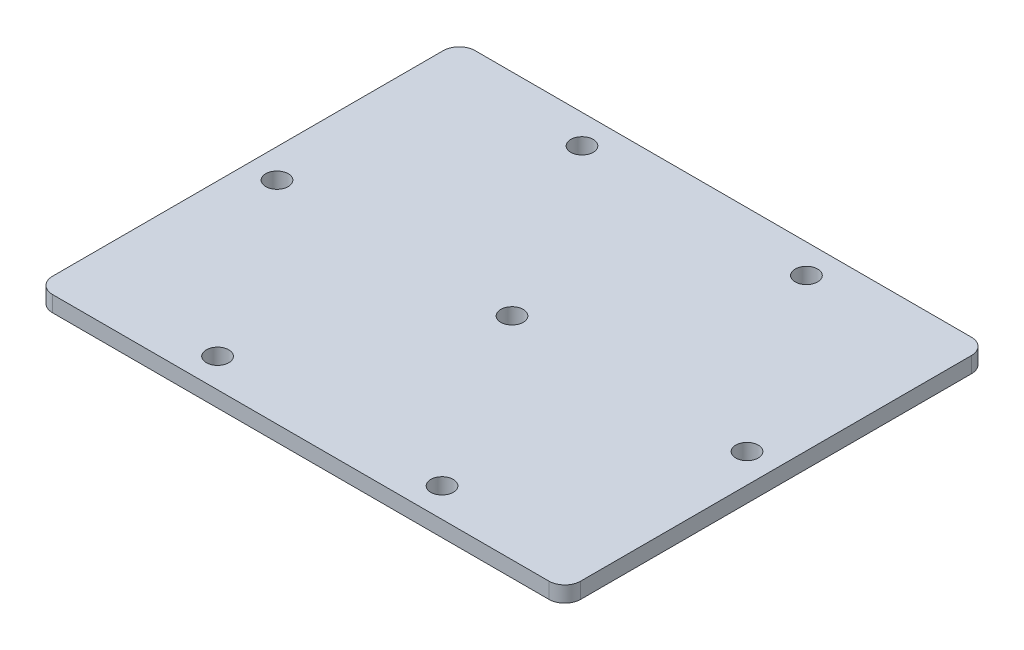
SolidWorks part; units mm, degrees
ref_plane "Front Plane" through (0, 0, 0) normal (0, 0, 1) x (1, 0, 0)
ref_plane "Top Plane" through (0, 0, 0) normal (0, 1, 0) x (1, 0, 0)
ref_plane "Right Plane" through (0, 0, 0) normal (1, 0, 0) x (0, 0, -1)
other "Configuration Table"
sketch "Sketch1" plane through (0, 0, 0) normal (0, 1, 0) x (1, 0, 0)
  line L1 (-100, -80) -> (100, -80)
  line L2 (-100, -80) -> (-100, 80)
  line L3 (-100, 80) -> (100, 80)
  line L4 (100, -80) -> (100, 80)
  line L5 (-100, -80) -> (100, 80) construction
  line L6 (-100, 80) -> (100, -80) construction
  point P0 (0, 0)
  dimension "D1" = 160
  dimension "D2" = 200
extrude "Boss-Extrude1" add sketch "Sketch1" along normal blind 6
fillet "Fillet1" radius 6 4 edges at (-100, 3, -80) (100, 3, -80) (100, 3, 80) (-100, 3, 80)
sketch "Sketch2" plane through (0, 6, 0) normal (0, 1, 0) x (1, 0, 0)
  line L0 (-138.2328, 0) -> (159.8736, 0) construction
  line L1 (0, 96.9307) -> (0, -97.5346) construction
  circle A0 centre (0, 0) radius 7.5
  circle A1 centre (-42.5, 69) radius 7.5
  circle A2 centre (42.5, 69) radius 7.5
  circle A3 centre (-89, 0) radius 7.5
  circle A4 centre (89, 0) radius 7.5
  circle A5 centre (-42.5, -69) radius 7.5
  circle A6 centre (42.5, -69) radius 7.5
  dimension "D1" = 15
  dimension "D2" = 15
  dimension "D3" = 15
  dimension "D4" = 15
  dimension "D5" = 15
  dimension "D6" = 15
  dimension "D7" = 15
  dimension "D8" = 85
  dimension "D9" = 138
  dimension "D10" = 178
hole_wizard "M10 Tapped Hole1" positions "Sketch3" profile "Sketch4" tap size "M10" standard "GB" end condition through all
sketch "Sketch3" plane through (0, 6, 0) normal (0, 1, 0) x (1, 0, 0)
  point P0 (0, 0)
  point P3 (42.5, 69)
  point P6 (-42.5, 69)
  point P9 (-89, 0)
  point P12 (89, 0)
  point P15 (42.5, -69)
  point P18 (-42.5, -69)
sketch "Sketch4" plane through (0, 6, 0) normal (1, 0, 0) x (0, 0, 1)
  line L0 (0, 0) -> (0, 6)
  line L1 (0, 6) -> (4.25, 6)
  line L2 (4.25, 6) -> (4.25, 0)
  line L5 (4.25, 0) -> (0, 0)
  line L11 (0, -6.35) -> (0, 107.95) construction
  dimension "通孔螺纹孔钻头直径" = 8.5
  dimension "通孔螺纹孔钻头深度" = 6
cosmetic thread "Cosmetic Thread1" parameters "D2"=10
cosmetic thread "Cosmetic Thread2" parameters "D2"=10
cosmetic thread "Cosmetic Thread3" parameters "D2"=10
cosmetic thread "Cosmetic Thread4" parameters "D2"=10
cosmetic thread "Cosmetic Thread5" parameters "D2"=10
cosmetic thread "Cosmetic Thread6" parameters "D2"=10
cosmetic thread "Cosmetic Thread7" parameters "D2"=10
